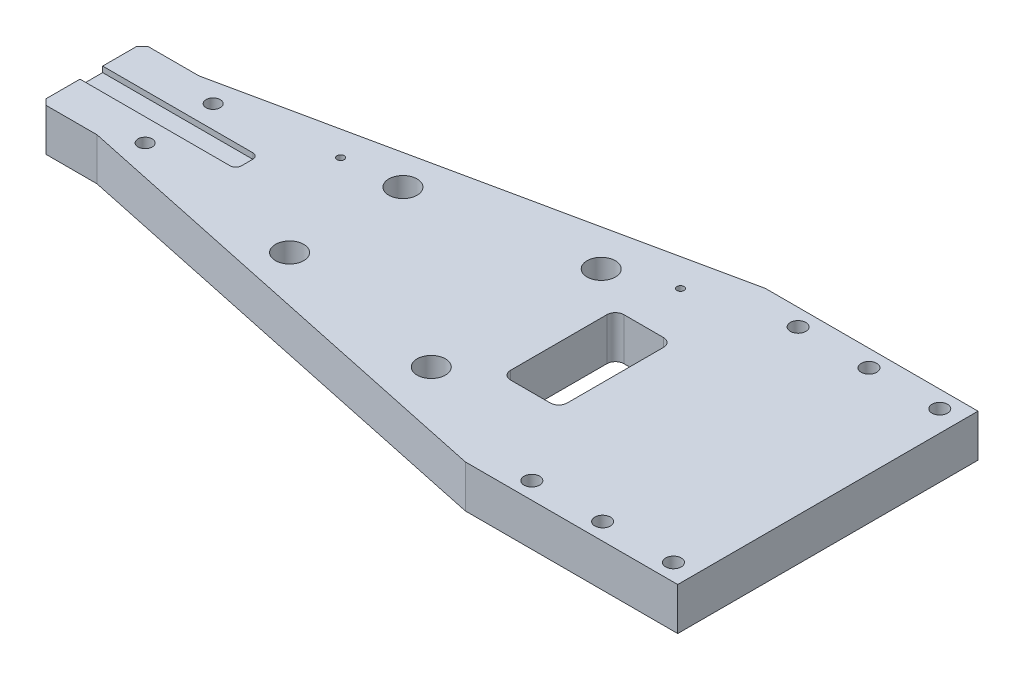
SolidWorks part; units mm, degrees
ref_plane "Front Plane" through (0, 0, 0) normal (0, 0, 1) x (1, 0, 0)
ref_plane "Top Plane" through (0, 0, 0) normal (0, 1, 0) x (1, 0, 0)
ref_plane "Right Plane" through (0, 0, 0) normal (1, 0, 0) x (0, 0, -1)
sketch "Sketch1" plane through (0, 0, 0) normal (0, 1, 0) x (1, 0, 0)
  line L1 (-130, 53) -> (130, 53)
  line L2 (-130, 53) -> (-130, -53)
  line L3 (-130, -53) -> (130, -53)
  line L4 (130, 53) -> (130, -53)
  line L5 (-130, 53) -> (130, -53) construction
  line L6 (-130, -53) -> (130, 53) construction
  point P0 (0, 0)
  dimension "D1" = 260
  dimension "D2" = 106
extrude "Boss-Extrude1" add sketch "Sketch1" along normal mid plane 15
sketch "Sketch2" plane through (0, 7.5, 0) normal (0, 1, 0) x (1, 0, 0)
  line L0 (55, 53) -> (-130, 53)
  line L1 (-130, 53) -> (-130, 18)
  line L2 (130, -53) -> (130, 53) construction
  line L3 (-130, -18) -> (-130, -53)
  line L4 (-130, -53) -> (55, -53)
  line L6 (-130, 53) -> (-130, -53) construction
  line L7 (130, 53) -> (-130, 53) construction
  line L8 (-130, -53) -> (130, -53) construction
  line L9 (0, 0) -> (-130, 0) construction
  line L10 (-130, -18) -> (-110, -18)
  line L11 (-110, -18) -> (55, -53)
  line L12 (-130, 18) -> (-110, 18)
  line L13 (-110, 18) -> (55, 53)
  dimension "D1" = 75
  dimension "D2" = 36
  dimension "D3" = 20
extrude "Cut-Extrude1" cut sketch "Sketch2" against normal through all
sketch "Sketch3" plane through (0, 7.5, 0) normal (0, 1, 0) x (1, 0, 0)
  line L0 (-130, 18) -> (-130, -18) construction
  line L1 (-130, 4) -> (-77, 4)
  line L2 (-130, 4) -> (-130, -4)
  line L3 (-130, -4) -> (-77, -4)
  line L4 (-75, 2) -> (-75, -2)
  line L5 (-130, 4) -> (-75, -4) construction
  line L6 (-130, -4) -> (-75, 4) construction
  line L7 (130, -53) -> (130, 53) construction
  arc A0 (-77, -4) -> (-75, -2) centre (-77, -2) ccw
  arc A1 (-75, 2) -> (-77, 4) centre (-77, 2) ccw
  point P0 (-102.5, 0)
  dimension "D3" = 2
  dimension "D1" = 8
  dimension "D2" = 205
extrude "Cut-Extrude2" cut sketch "Sketch3" against normal blind 2
hole_wizard "M6 Tapped Hole1" positions "Sketch8" profile "Sketch7" tap size "M6" standard "Gb" end condition through all
sketch "Sketch8" plane through (0, 7.5, 0) normal (0, 1, 0) x (1, 0, 0)
  line L0 (0, 0) -> (-140.6405, 0) construction
  line L3 (130, -53) -> (130, 53) construction
  point P0 (-99, 12)
  point P2 (-99, -12)
  dimension "D1" = 24
  dimension "D2" = 229
sketch "Sketch7" plane through (-99, 7.5, -12) normal (1, 0, 0) x (0, 0, 1)
  line L0 (0, 0) -> (0, 15)
  line L1 (0, 15) -> (2.5, 15)
  line L2 (2.5, 15) -> (2.5, 0)
  line L5 (2.5, 0) -> (0, 0)
  line L11 (0, -6.35) -> (0, 107.95) construction
  dimension "通孔螺纹孔钻头直径" = 5
  dimension "通孔螺纹孔钻头深度" = 15
cosmetic thread "Hole Thread1" parameters "D2"=6
cosmetic thread "Hole Thread2" parameters "D2"=6
sketch "Sketch9" plane through (0, 7.5, 0) normal (0, 1, 0) x (1, 0, 0)
  line L1 (35, 20) -> (55, 20)
  line L2 (35, 20) -> (35, -20)
  line L3 (35, -20) -> (55, -20)
  line L4 (55, 20) -> (55, -20)
  line L5 (35, 20) -> (55, -20) construction
  line L6 (35, -20) -> (55, 20) construction
  line L7 (130, -53) -> (130, 53) construction
  point P0 (45, 0)
  dimension "D1" = 20
  dimension "D2" = 40
  dimension "D3" = 85
extrude "Cut-Extrude4" cut sketch "Sketch9" against normal through all
fillet "Fillet5" radius 3 4 edges at (55, 0, 20) (55, 0, -20) (35, 0, -20) (35, 0, 20)
hole_wizard "Hole size per socket head cap screw type1" positions "Sketch11" profile "Sketch10" counterbore size "M5" standard "Gb" end condition through all
sketch "Sketch11" plane through (0, -7.5, 0) normal (0, -1, 0) x (-1, 0, 0)
  line L0 (0, 0) -> (-141.1083, 0) construction
  line L2 (-130, -53) -> (-130, 53) construction
  point P0 (-122.5, -47)
  point P3 (-97.5, -47)
  point P6 (-72.5, -47)
  point P9 (-72.5, 47)
  point P11 (-97.5, 47)
  point P14 (-122.5, 47)
  dimension "D1" = 94
  dimension "D2" = 7.5
  dimension "D3" = 25
  dimension "D4" = 25
sketch "Sketch10" plane through (122.5, -7.5, 47) normal (1, 0, 0) x (0, 0, -1)
  line L0 (0, 0) -> (0, 15)
  line L1 (0, 15) -> (2.75, 15)
  line L3 (2.75, 15) -> (2.75, 6)
  line L4 (2.75, 6) -> (5, 6)
  line L5 (5, 6) -> (5, 0)
  line L7 (5, 0) -> (0, 0)
  line L11 (0, -6.35) -> (0, 107.95) construction
  dimension "通孔孔直径" = 5.5
  dimension "通孔孔深度" = 15
  dimension "柱形沉头孔直径" = 10
  dimension "柱形沉头孔深度" = 6
chamfer "Chamfer1" distance 2 angle 45 2 edges at (-130, 0, 18) (-130, 0, -18)
hole_wizard "M3 Tapped Hole1" positions "Sketch18" profile "Sketch17" tap size "M3" standard "Gb"
sketch "Sketch18" plane through (0, 7.5, 0) normal (0, 1, 0) x (1, 0, 0)
  line L0 (130, 53) -> (55, 53) construction
  line L1 (130, -53) -> (130, 53) construction
  point P0 (40, 38)
  point P7 (-60, 18)
  dimension "D1" = 15
  dimension "D2" = 90
  dimension "D3" = 100
  dimension "D4" = 35
sketch "Sketch17" plane through (40, 7.5, -38) normal (1, 0, 0) x (0, 0, 1)
  line L0 (0, 0) -> (0, 8.2511)
  line L1 (0, 8.2511) -> (1.25, 7.5)
  line L2 (1.25, 7.5) -> (1.25, 0)
  line L5 (1.25, 0) -> (0, 0)
  line L10 (0, 8.2511) -> (-1.25, 7.5) construction
  line L11 (0, -6.35) -> (0, 107.95) construction
  dimension "螺纹孔钻头直径" = 2.5
  dimension "螺纹孔钻头深度" = 7.5
  dimension "导头角度" = 118
cosmetic thread "Hole Thread3" parameters "D1"=6, "D2"=3
cosmetic thread "Hole Thread4" parameters "D1"=6, "D2"=3
hole_wizard "Ø10.0 (10) Diameter Hole1" positions "Sketch20" profile "Sketch19" hole size "Ø10.0" standard "Gb" end condition through all
sketch "Sketch20" plane through (0, 7.5, 0) normal (0, 1, 0) x (1, 0, 0)
  line L0 (0, 0) -> (-61.4002, 0) construction
  line L2 (130, -53) -> (130, 53) construction
  point P0 (-40, 20)
  point P2 (-40, -20)
  point P4 (20, -30)
  point P6 (20, 30)
  dimension "D1" = 40
  dimension "D2" = 60
  dimension "D3" = 60
  dimension "D4" = 110
sketch "Sketch19" plane through (-40, 7.5, -20) normal (1, 0, 0) x (0, 0, 1)
  line L0 (0, 0) -> (0, 15)
  line L1 (0, 15) -> (5, 15)
  line L2 (5, 15) -> (5, 0)
  line L5 (5, 0) -> (0, 0)
  line L11 (0, -6.35) -> (0, 107.95) construction
  dimension "通孔孔直径" = 10
  dimension "通孔孔深度" = 15
